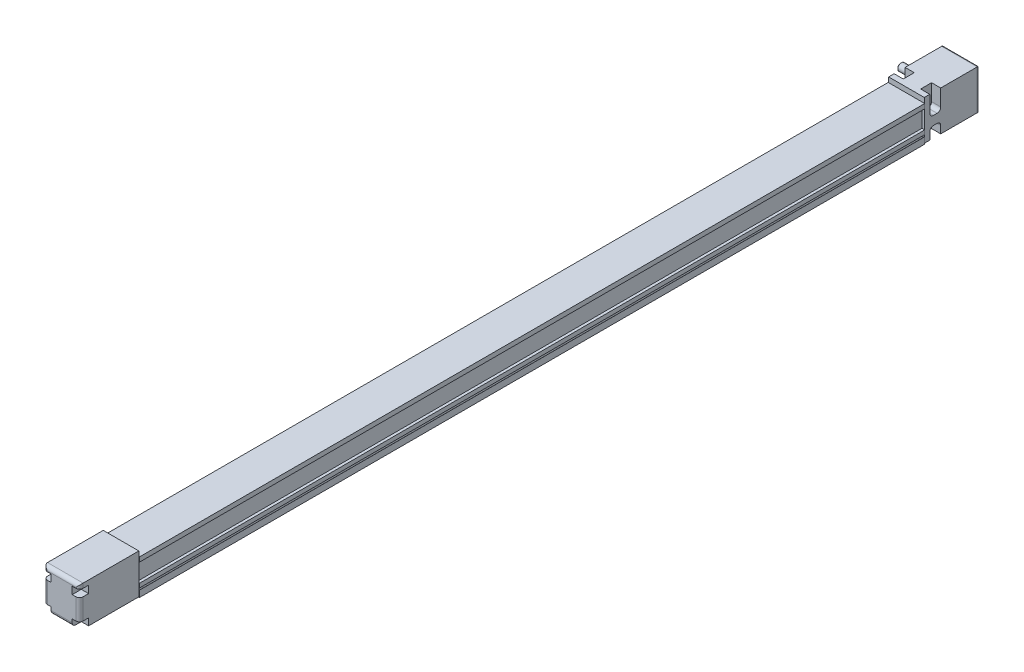
from build123d import *

# Parameters (mm, degrees)
EXTRUDE_473_DEPTH      = 860
SKETCH_2_W             = 39
SKETCH_2_H             = 43.557766586
EXTRUDE_1_DEPTH        = 65
FILLET_2_R             = 4
SKETCH_3_W             = 8
SKETCH_3_H             = 8
CUT_EXTRUDE_1_DEPTH    = 10
SKETCH_4_W             = 39
SKETCH_4_H             = 43.557766586
EXTRUDE_3_DEPTH        = 60
FILLET_4_R             = 2
CUT_EXTRUDE_2_DEPTH    = 10
CUT_EXTRUDE_START      = -10
CUT_EXTRUDE_3_DEPTH    = 10
HOLE_WIZARD_M4_1_D     = 3.3
HOLE_WIZARD_M4_1_DEPTH = 10.1
HOLE_WIZARD_M4_1_TIP   = 0.991420021
SKETCH_13_R            = 18.5
CUT_EXTRUDE_4_DEPTH    = 3
SKETCH_14_R            = 4
EXTRUDE_5_DEPTH        = 28
CHAMFER_1_SIZE         = 1


with BuildPart() as part:
    # 草图1 → Extrude 473 (new body)
    with BuildSketch(Plane.XY):
        Polygon((0, 0), (40, 0), (40, 7), (38, 5.057766586), (38, 9.057766586), (40, 9.057766586), (40, 13.557766586), (37, 13.557766586), (37, 33.557766586), (40, 33.557766586), (40, 38.557766586), (0, 38.557766586), (0, 33.557766586), (3, 33.557766586), (3, 13.557766586), (0, 13.557766586), (0, 9.057766586), (2, 9.057766586), (2, 5.057766586), (0, 7), align=None)
    extrude(amount=EXTRUDE_473_DEPTH)

    # 草图2 → 凸台-拉伸1 (add)
    with BuildSketch(Plane.XY.offset(860)):
        with Locations((20, 22.278883293)):
            Rectangle(SKETCH_2_W, SKETCH_2_H)
    extrude(amount=EXTRUDE_1_DEPTH)

    # 圆角2
    fillet_2_edges = [part.edges().sort_by_distance(p)[0] for p in [
        (0.5, 22.278883293, 925),
        (20, 0.5, 925),
        (39.5, 22.278883293, 925),
        (20, 44.057766586, 925),
    ]]
    fillet(fillet_2_edges, radius=FILLET_2_R)

    # 草图3 → 切除-拉伸1 (cut)
    with BuildSketch(Plane.XY.offset(925)):
        with Locations((4.5, 35.134037638)):
            Rectangle(SKETCH_3_W, SKETCH_3_H)
        with Locations((35.5, 4.134037638)):
            Rectangle(SKETCH_3_W, SKETCH_3_H)
        with Locations((35.5, 35.134037638)):
            Rectangle(SKETCH_3_W, SKETCH_3_H)
        with Locations((4.5, 4.134037638)):
            Rectangle(SKETCH_3_W, SKETCH_3_H)
    extrude(amount=-CUT_EXTRUDE_1_DEPTH, mode=Mode.SUBTRACT)

    # 草图4 → 凸台-拉伸3 (add)
    with BuildSketch(Plane(origin=(0, 0, 0), x_dir=(-1, 0, 0), z_dir=(0, 0, -1))):
        with Locations((-20, 22.278883293)):
            Rectangle(SKETCH_4_W, SKETCH_4_H)
    extrude(amount=EXTRUDE_3_DEPTH)

    # 圆角4
    fillet_4_edges = [part.edges().sort_by_distance(p)[0] for p in [
        (39.5, 22.278883293, -60),
        (20, 0.5, -60),
        (0.5, 22.278883293, -60),
        (20, 44.057766586, -60),
    ]]
    fillet(fillet_4_edges, radius=FILLET_4_R)

    # 草图5 → 切除-拉伸2 (cut)
    with BuildSketch(Plane.ZY.offset(-0.5)):
        with BuildLine():
            Line((-18, 44.057766586), (-6, 44.057766586))
            Line((-6, 44.057766586), (-6, 26.057766586))
            ThreePointArc((-6, 26.057766586), (-7.171572875, 23.229339461), (-10, 22.057766586))
            Line((-10, 22.057766586), (-14, 22.057766586))
            ThreePointArc((-14, 22.057766586), (-16.828427125, 23.229339461), (-18, 26.057766586))
            Line((-18, 26.057766586), (-18, 44.057766586))
        make_face()
        with BuildLine():
            Line((-14, 12.5), (-10, 12.5))
            ThreePointArc((-10, 12.5), (-7.171572875, 11.328427125), (-6, 8.5))
            Line((-6, 8.5), (-6, 0.5))
            Line((-6, 0.5), (-18, 0.5))
            Line((-18, 0.5), (-18, 8.5))
            ThreePointArc((-18, 8.5), (-16.828427125, 11.328427125), (-14, 12.5))
        make_face()
    extrude(amount=-CUT_EXTRUDE_2_DEPTH, mode=Mode.SUBTRACT)

    # 草图7 → 切除-拉伸3 (cut)
    with BuildSketch(Plane(origin=(39.5, 0, 0), x_dir=(0, 0, -1), z_dir=(1, 0, 0)).offset(CUT_EXTRUDE_START)):
        with BuildLine():
            Line((6, 44.057766586), (18, 44.057766586))
            Line((18, 44.057766586), (18, 26.057766586))
            ThreePointArc((18, 26.057766586), (16.828427125, 23.229339461), (14, 22.057766586))
            Line((14, 22.057766586), (10, 22.057766586))
            ThreePointArc((10, 22.057766586), (7.171572875, 23.229339461), (6, 26.057766586))
            Line((6, 26.057766586), (6, 44.057766586))
        make_face()
        with BuildLine():
            Line((10, 12.5), (14, 12.5))
            ThreePointArc((14, 12.5), (16.828427125, 11.328427125), (18, 8.5))
            Line((18, 8.5), (18, 0.5))
            Line((18, 0.5), (6, 0.5))
            Line((6, 0.5), (6, 8.5))
            ThreePointArc((6, 8.5), (7.171572875, 11.328427125), (10, 12.5))
        make_face()
    extrude(amount=CUT_EXTRUDE_3_DEPTH, mode=Mode.SUBTRACT)

    # M4 螺纹孔1
    with Locations(Plane.ZY.offset(-0.5)):
        with Locations((-22, 6.557766586), (-54, 6.557766586), (-22, 38.557766586), (-54, 38.557766586)):
            Hole(HOLE_WIZARD_M4_1_D / 2, depth=HOLE_WIZARD_M4_1_DEPTH)
            with Locations((0, 0, -(HOLE_WIZARD_M4_1_DEPTH + HOLE_WIZARD_M4_1_TIP / 2))):  # 118° drill point
                Cone(0, HOLE_WIZARD_M4_1_D / 2, HOLE_WIZARD_M4_1_TIP, mode=Mode.SUBTRACT)

    # 草图13 → 切除-拉伸4 (cut)
    with BuildSketch(Plane.ZY.offset(-0.5)):
        with Locations((-38, 22.557766586)):
            Circle(SKETCH_13_R)
    extrude(amount=-CUT_EXTRUDE_4_DEPTH, mode=Mode.SUBTRACT)

    # 草图14 → 凸台-拉伸5 (add)
    with BuildSketch(Plane.ZY.offset(-3.5)):
        with Locations((-38, 22.557766586)):
            Circle(SKETCH_14_R)
    extrude(amount=EXTRUDE_5_DEPTH)

    # 倒角1
    chamfer_1_edges = [part.edges().sort_by_distance(p)[0] for p in [
        (-24.5, 22.557766586, -42),
    ]]
    chamfer(chamfer_1_edges, length=CHAMFER_1_SIZE)


solid = part.part
